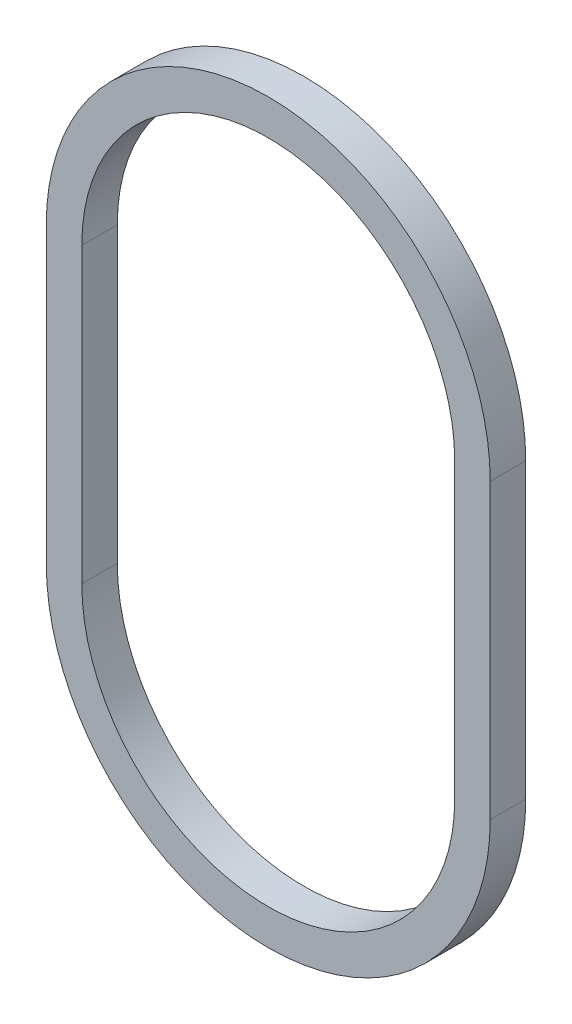
SolidWorks part; units mm, degrees
ref_plane "前视基准面" through (0, 0, 0) normal (0, 0, 1) x (1, 0, 0)
ref_plane "上视基准面" through (0, 0, 0) normal (0, 1, 0) x (1, 0, 0)
ref_plane "右视基准面" through (0, 0, 0) normal (1, 0, 0) x (0, 0, -1)
sketch "草图1" plane through (0, 0, 0) normal (0, 0, 1) x (1, 0, 0)
  line L0 (-25, 16.5) -> (-25, -16.5)
  line L1 (25, 16.5) -> (25, -16.5)
  line L2 (-21, 16.5) -> (-21, -16.5)
  line L4 (21, 16.5) -> (21, -16.5)
  arc A0 (21, 16.5) -> (-21, 16.5) centre (0, 16.5) ccw
  arc A1 (21, -16.5) -> (-21, -16.5) centre (0, -16.5) cw
  arc A2 (25, 16.5) -> (-25, 16.5) centre (0, 16.5) ccw
  arc A3 (25, -16.5) -> (-25, -16.5) centre (0, -16.5) cw
  point P0 (0, 0)
  dimension "D1" = 21
  dimension "D2" = 21
  dimension "D3" = 33
  dimension "D4" = 4
extrude "凸台-拉伸1" add sketch "草图1" along normal blind 4
